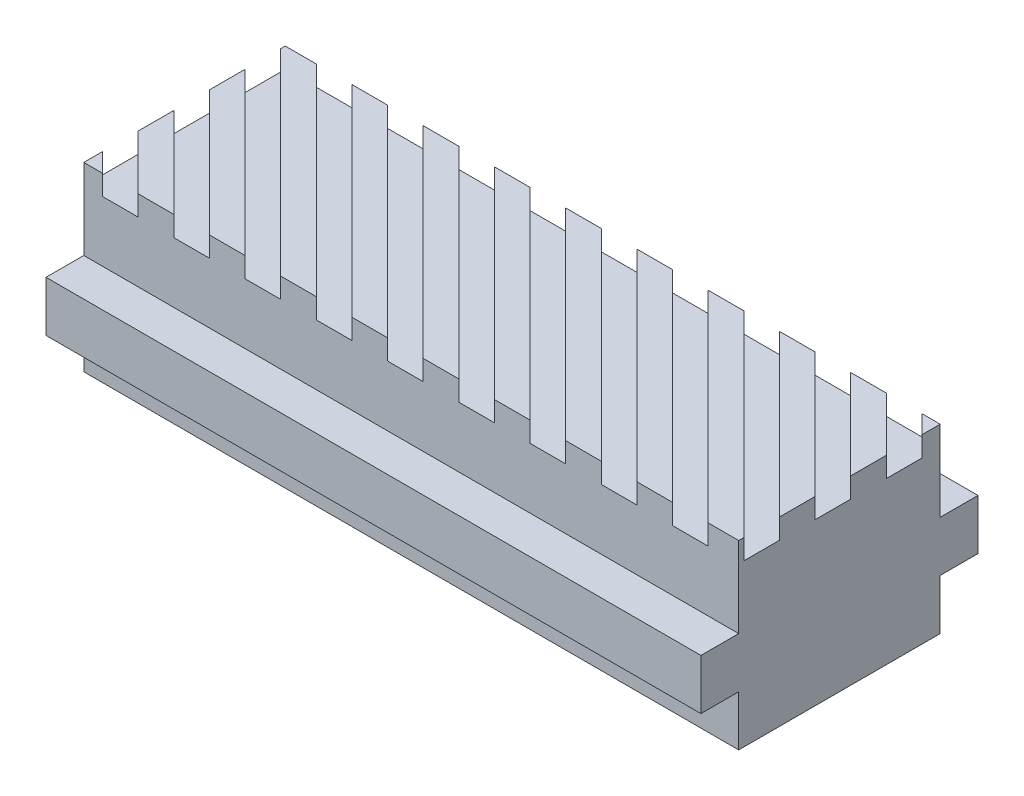
from build123d import *

# Parameters (mm, degrees)
SKETCH1_W           = 180
SKETCH1_H           = 40
BOSS_EXTRUDE1_DEPTH = 6
CUT_EXTRUDE2_DEPTH  = 4
SKETCH6_W           = 180
SKETCH6_H           = 40
BOSS_EXTRUDE3_DEPTH = 30
SKETCH7_W           = 50
SKETCH7_H           = 40
CUT_EXTRUDE3_DEPTH  = 40
SKETCH8_W           = 55
SKETCH8_H           = 10
BOSS_EXTRUDE4_DEPTH = 130
SKETCH9_R           = 7.5
CUT_EXTRUDE4_DEPTH  = 25


with BuildPart() as part:
    # Sketch1 → Boss-Extrude1 (new body)
    with BuildSketch(Plane(origin=(0, 0, 0), x_dir=(1, 0, 0), z_dir=(0, 1, 0))):
        Rectangle(SKETCH1_W, SKETCH1_H)
    extrude(amount=BOSS_EXTRUDE1_DEPTH)

    # Sketch5 → Cut-Extrude2 (cut)
    with BuildSketch(Plane(origin=(0, 6, 0), x_dir=(1, 0, 0), z_dir=(0, 1, 0))):
        with BuildLine():
            Line((-105.561478508, 98.797927369), (119.027484656, -125.791035795))
            ThreePointArc((119.027484656, -125.791035795), (119.027484656, -129.326569701), (115.49195075, -129.326569701))
            Line((115.49195075, -129.326569701), (-109.097012414, 95.262393463))
            ThreePointArc((-109.097012414, 95.262393463), (-109.097012414, 98.797927369), (-105.561478508, 98.797927369))
        make_face()
        with BuildLine():
            Line((-102.025944602, 102.333461275), (122.563018562, -122.255501889))
            ThreePointArc((122.563018562, -122.255501889), (126.098552468, -122.255501889), (126.098552468, -118.719967983))
            Line((126.098552468, -118.719967983), (-98.490410696, 105.868995181))
            ThreePointArc((-98.490410696, 105.868995181), (-102.025944602, 105.868995181), (-102.025944602, 102.333461275))
        make_face()
        with BuildLine():
            Line((-94.95487679, 109.404529087), (129.634086374, -115.184434077))
            ThreePointArc((129.634086374, -115.184434077), (133.16962028, -115.184434077), (133.16962028, -111.648900171))
            Line((133.16962028, -111.648900171), (-91.419342885, 112.940062993))
            ThreePointArc((-91.419342885, 112.940062993), (-94.95487679, 112.940062993), (-94.95487679, 109.404529087))
        make_face()
        with BuildLine():
            Line((-87.883808979, 116.475596899), (136.705154185, -108.113366265))
            ThreePointArc((136.705154185, -108.113366265), (140.240688091, -108.113366265), (140.240688091, -104.577832359))
            Line((140.240688091, -104.577832359), (-84.348275073, 120.011130805))
            ThreePointArc((-84.348275073, 120.011130805), (-87.883808979, 120.011130805), (-87.883808979, 116.475596899))
        make_face()
        with BuildLine():
            Line((-80.812741167, 123.546664711), (143.776221997, -101.042298453))
            ThreePointArc((143.776221997, -101.042298453), (147.311755903, -101.042298453), (147.311755903, -97.506764547))
            Line((147.311755903, -97.506764547), (-77.277207261, 127.082198617))
            ThreePointArc((-77.277207261, 127.082198617), (-80.812741167, 127.082198617), (-80.812741167, 123.546664711))
        make_face()
        with BuildLine():
            Line((-73.741673355, 130.617732523), (150.847289809, -93.971230641))
            ThreePointArc((150.847289809, -93.971230641), (154.382823715, -93.971230641), (154.382823715, -90.435696735))
            Line((154.382823715, -90.435696735), (-70.206139449, 134.153266429))
            ThreePointArc((-70.206139449, 134.153266429), (-73.741673355, 134.153266429), (-73.741673355, 130.617732523))
        make_face()
        with BuildLine():
            Line((-66.670605543, 137.688800335), (157.918357621, -86.900162829))
            ThreePointArc((157.918357621, -86.900162829), (161.453891527, -86.900162829), (161.453891527, -83.364628923))
            Line((161.453891527, -83.364628923), (-63.135071637, 141.224334241))
            ThreePointArc((-63.135071637, 141.224334241), (-66.670605543, 141.224334241), (-66.670605543, 137.688800335))
        make_face()
        with BuildLine():
            Line((-59.599537731, 144.759868147), (164.989425433, -79.829095018))
            ThreePointArc((164.989425433, -79.829095018), (168.524959339, -79.829095018), (168.524959339, -76.293561112))
            Line((168.524959339, -76.293561112), (-56.064003825, 148.295402052))
            ThreePointArc((-56.064003825, 148.295402052), (-59.599537731, 148.295402052), (-59.599537731, 144.759868147))
        make_face()
        with BuildLine():
            Line((-52.528469919, 151.830935958), (172.060493245, -72.758027206))
            ThreePointArc((172.060493245, -72.758027206), (175.596027151, -72.758027206), (175.596027151, -69.2224933))
            Line((175.596027151, -69.2224933), (-48.992936013, 155.366469864))
            ThreePointArc((-48.992936013, 155.366469864), (-52.528469919, 155.366469864), (-52.528469919, 151.830935958))
        make_face()
        with BuildLine():
            Line((-45.457402107, 158.90200377), (179.131561057, -65.686959394))
            ThreePointArc((179.131561057, -65.686959394), (182.667094963, -65.686959394), (182.667094963, -62.151425488))
            Line((182.667094963, -62.151425488), (-41.921868201, 162.437537676))
            ThreePointArc((-41.921868201, 162.437537676), (-45.457402107, 162.437537676), (-45.457402107, 158.90200377))
        make_face()
        with BuildLine():
            Line((-116.168080226, 88.191325652), (108.420882938, -136.397637512))
            ThreePointArc((108.420882938, -136.397637512), (111.956416844, -136.397637512), (111.956416844, -132.862103607))
            Line((111.956416844, -132.862103607), (-112.63254632, 91.726859558))
            ThreePointArc((-112.63254632, 91.726859558), (-116.168080226, 91.726859558), (-116.168080226, 88.191325652))
        make_face()
        with BuildLine():
            Line((-123.239148038, 81.12025784), (101.349815126, -143.468705324))
            ThreePointArc((101.349815126, -143.468705324), (104.885349032, -143.468705324), (104.885349032, -139.933171418))
            Line((104.885349032, -139.933171418), (-119.703614132, 84.655791746))
            ThreePointArc((-119.703614132, 84.655791746), (-123.239148038, 84.655791746), (-123.239148038, 81.12025784))
        make_face()
        with BuildLine():
            Line((-130.31021585, 74.049190028), (94.278747314, -150.539773136))
            ThreePointArc((94.278747314, -150.539773136), (97.81428122, -150.539773136), (97.81428122, -147.00423923))
            Line((97.81428122, -147.00423923), (-126.774681944, 77.584723934))
            ThreePointArc((-126.774681944, 77.584723934), (-130.31021585, 77.584723934), (-130.31021585, 74.049190028))
        make_face()
        with BuildLine():
            Line((-137.381283662, 66.978122216), (87.207679502, -157.610840948))
            ThreePointArc((87.207679502, -157.610840948), (90.743213408, -157.610840948), (90.743213408, -154.075307042))
            Line((90.743213408, -154.075307042), (-133.845749756, 70.513656122))
            ThreePointArc((-133.845749756, 70.513656122), (-137.381283662, 70.513656122), (-137.381283662, 66.978122216))
        make_face()
        with BuildLine():
            Line((-144.452351474, 59.907054404), (80.136611691, -164.68190876))
            ThreePointArc((80.136611691, -164.68190876), (83.672145596, -164.68190876), (83.672145596, -161.146374854))
            Line((83.672145596, -161.146374854), (-140.916817568, 63.44258831))
            ThreePointArc((-140.916817568, 63.44258831), (-144.452351474, 63.44258831), (-144.452351474, 59.907054404))
        make_face()
        with BuildLine():
            Line((-151.523419285, 52.835986592), (73.065543879, -171.752976572))
            ThreePointArc((73.065543879, -171.752976572), (76.601077785, -171.752976572), (76.601077785, -168.217442666))
            Line((76.601077785, -168.217442666), (-147.987885379, 56.371520498))
            ThreePointArc((-147.987885379, 56.371520498), (-151.523419285, 56.371520498), (-151.523419285, 52.835986592))
        make_face()
        with BuildLine():
            Line((-158.594487097, 45.76491878), (65.994476067, -178.824044384))
            ThreePointArc((65.994476067, -178.824044384), (69.530009973, -178.824044384), (69.530009973, -175.288510478))
            Line((69.530009973, -175.288510478), (-155.058953191, 49.300452686))
            ThreePointArc((-155.058953191, 49.300452686), (-158.594487097, 49.300452686), (-158.594487097, 45.76491878))
        make_face()
    extrude(amount=-CUT_EXTRUDE2_DEPTH, mode=Mode.SUBTRACT)

    # Sketch6 → Boss-Extrude3 (add)
    with BuildSketch(Plane.XZ):
        Rectangle(SKETCH6_W, SKETCH6_H)
    extrude(amount=BOSS_EXTRUDE3_DEPTH)

    # Sketch7 → Cut-Extrude3 (cut)
    with BuildSketch(Plane.XZ.offset(30)):
        with Locations((-65, 0)):
            Rectangle(SKETCH7_W, SKETCH7_H)
    extrude(amount=-CUT_EXTRUDE3_DEPTH, mode=Mode.SUBTRACT)

    # Sketch8 → Boss-Extrude4 (add, through all)
    with BuildSketch(Plane(origin=(90, 0, 0), x_dir=(0, 0, -1), z_dir=(1, 0, 0))):
        with Locations((0, -15)):
            Rectangle(SKETCH8_W, SKETCH8_H)
    extrude(amount=-BOSS_EXTRUDE4_DEPTH)

    # Sketch9 → Cut-Extrude4 (cut)
    with BuildSketch(Plane.XZ.offset(30)):
        with Locations(Location((60, 0, 0), (0, 0, 270))):
            Circle(SKETCH9_R)
        with Locations(Location((-10, 0, 0), (0, 0, 270))):
            Circle(SKETCH9_R)
    extrude(amount=-CUT_EXTRUDE4_DEPTH, mode=Mode.SUBTRACT)


solid = part.part
